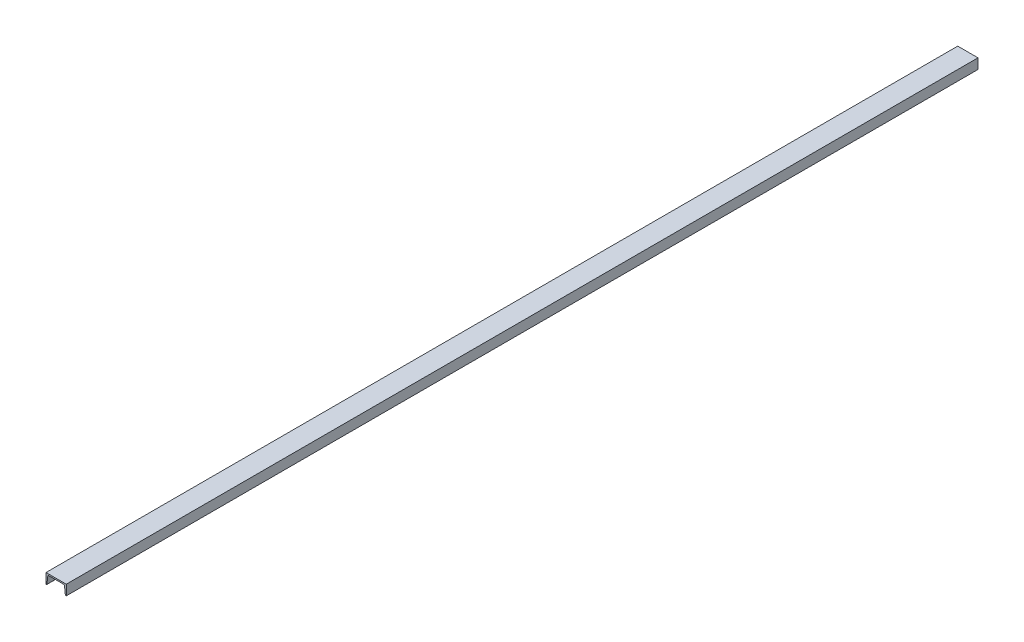
SolidWorks part; units mm, degrees
material "普通碳钢"
ref_plane "Front Plane" through (0, 0, 0) normal (0, 0, 1) x (1, 0, 0)
ref_plane "Top Plane" through (0, 0, 0) normal (0, 1, 0) x (1, 0, 0)
ref_plane "Right Plane" through (0, 0, 0) normal (1, 0, 0) x (0, 0, -1)
sketch "Sketch1" plane through (0, 0, 0) normal (0, 0, 1) x (1, 0, 0)
  line L0 (0, 0) -> (0, 50)
  line L1 (0, 50) -> (100, 50)
  line L2 (100, 50) -> (100, 0)
  line L3 (0, 0) -> (2.5485, 0)
  line L4 (4.5356, 1.7732) -> (8.7527, 38.7239)
  line L5 (13.7205, 43.1569) -> (86.2795, 43.1569)
  line L6 (50, 50) -> (50, 36.5447) construction
  line L7 (100, 0) -> (97.4515, 0)
  line L8 (95.4644, 1.7732) -> (91.2473, 38.7239)
  arc A0 (8.7527, 38.7239) -> (13.7205, 43.1569) centre (13.7205, 38.1569) cw
  arc A1 (4.5356, 1.7732) -> (2.5485, 0) centre (2.5485, 2) cw
  arc A2 (91.2473, 38.7239) -> (86.2795, 43.1569) centre (86.2795, 38.1569) ccw
  arc A3 (95.4644, 1.7732) -> (97.4515, 0) centre (97.4515, 2) ccw
  point P15 (50, 43.1569)
  dimension "D4" = 5
  dimension "D5" = 2
  dimension "D1" = 100
  dimension "D3" = 50
extrude "Boss-Extrude1" add sketch "Sketch1" along normal blind 4500
